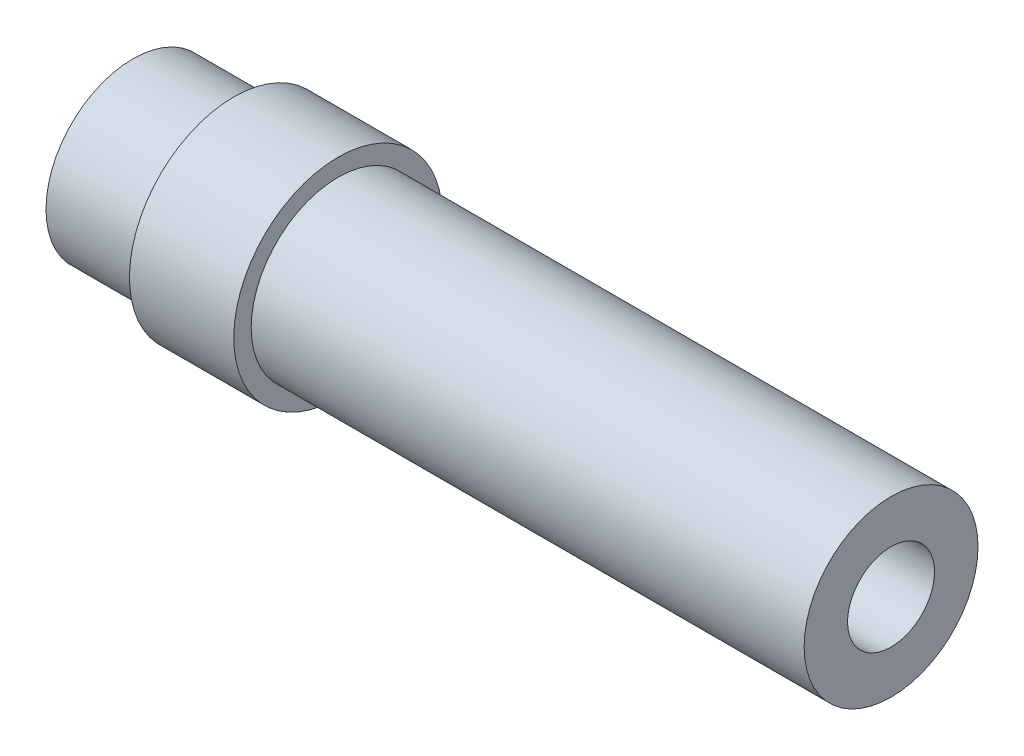
from build123d import *

# Parameters (mm, degrees)
M3_TAPPED_HOLE1_D               = 2.5
M3_TAPPED_HOLE1_DEPTH           = 8
M3_TAPPED_HOLE1_TIP             = 0.751075774
M3_TAPPED_HOLE1_ON_FACE_2_D     = 2.5
M3_TAPPED_HOLE1_ON_FACE_2_DEPTH = 8
M3_TAPPED_HOLE1_ON_FACE_2_TIP   = 0.751075774


with BuildPart() as part:
    # Sketch1 → Revolve1 (revolve)
    with BuildSketch(Plane.XY):
        Polygon((22.305681316, -2.5), (0.505681316, -2.5), (0.505681316, 0), (3.405681316, 0), (3.405681316, 0.5), (6.405681316, 0.5), (6.405681316, 0), (22.305681316, 0), align=None)
    revolve(axis=Axis((22.305681316, -2.5, 0), (-1, 0, 0)))

    # M3 Tapped Hole1
    with Locations(Plane(origin=(0.505681316, -2.5, 0), x_dir=(0, 0, -1), z_dir=(-1, 0, 0))):
        with Locations((0, 0)):
            Hole(M3_TAPPED_HOLE1_D / 2, depth=M3_TAPPED_HOLE1_DEPTH)
            with Locations((0, 0, -(M3_TAPPED_HOLE1_DEPTH + M3_TAPPED_HOLE1_TIP / 2))):  # 118° drill point
                Cone(0, M3_TAPPED_HOLE1_D / 2, M3_TAPPED_HOLE1_TIP, mode=Mode.SUBTRACT)

    # M3 Tapped Hole1 on face 2
    with Locations(Plane(origin=(22.305681316, -2.5, 0), x_dir=(0, 0, 1), z_dir=(1, 0, 0))):
        with Locations((0, 0)):
            Hole(M3_TAPPED_HOLE1_ON_FACE_2_D / 2, depth=M3_TAPPED_HOLE1_ON_FACE_2_DEPTH)
            with Locations((0, 0, -(M3_TAPPED_HOLE1_ON_FACE_2_DEPTH + M3_TAPPED_HOLE1_ON_FACE_2_TIP / 2))):  # 118° drill point
                Cone(0, M3_TAPPED_HOLE1_ON_FACE_2_D / 2, M3_TAPPED_HOLE1_ON_FACE_2_TIP, mode=Mode.SUBTRACT)


solid = part.part
